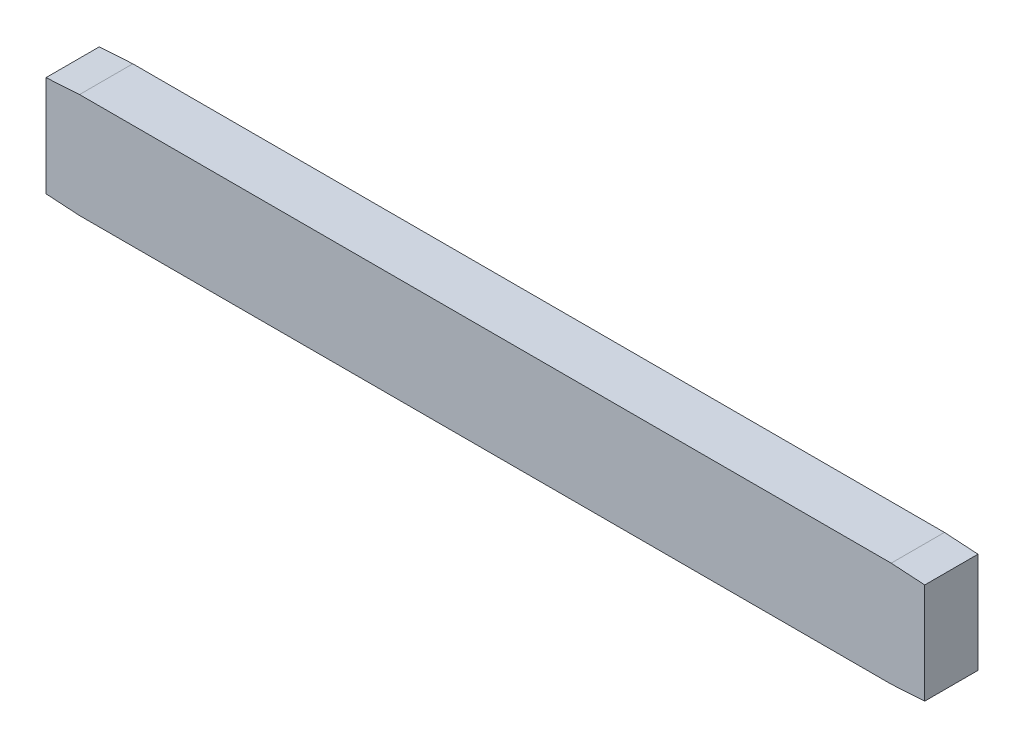
from build123d import *

# Parameters (mm, degrees)
SKETCH1_W          = 209.55
SKETCH1_H          = 25
EXTRUDE1_DEPTH     = 6.35
CUT_EXTRUDE1_DEPTH = 107.279540011


with BuildPart() as part:
    # Sketch1 → Extrude1 (new, symmetric)
    with BuildSketch(Plane.XY):
        Rectangle(SKETCH1_W, SKETCH1_H)
    extrude(amount=EXTRUDE1_DEPTH, both=True)

    # Sketch2 → Cut-Extrude1 (cut, through all)
    with BuildSketch(Plane.XY.offset(6.35)):
        Polygon((-104.775, 12), (-96.775, 12.5), (-104.775, 12.5), align=None)
        Polygon((96.775, 12.5), (104.775, 12.5), (104.775, 12), align=None)
        Polygon((104.775, -12.5), (104.775, -12), (96.775, -12.5), align=None)
        Polygon((-96.775, -12.5), (-104.775, -12.5), (-104.775, -12), align=None)
    extrude(amount=-CUT_EXTRUDE1_DEPTH, mode=Mode.SUBTRACT)


solid = part.part
